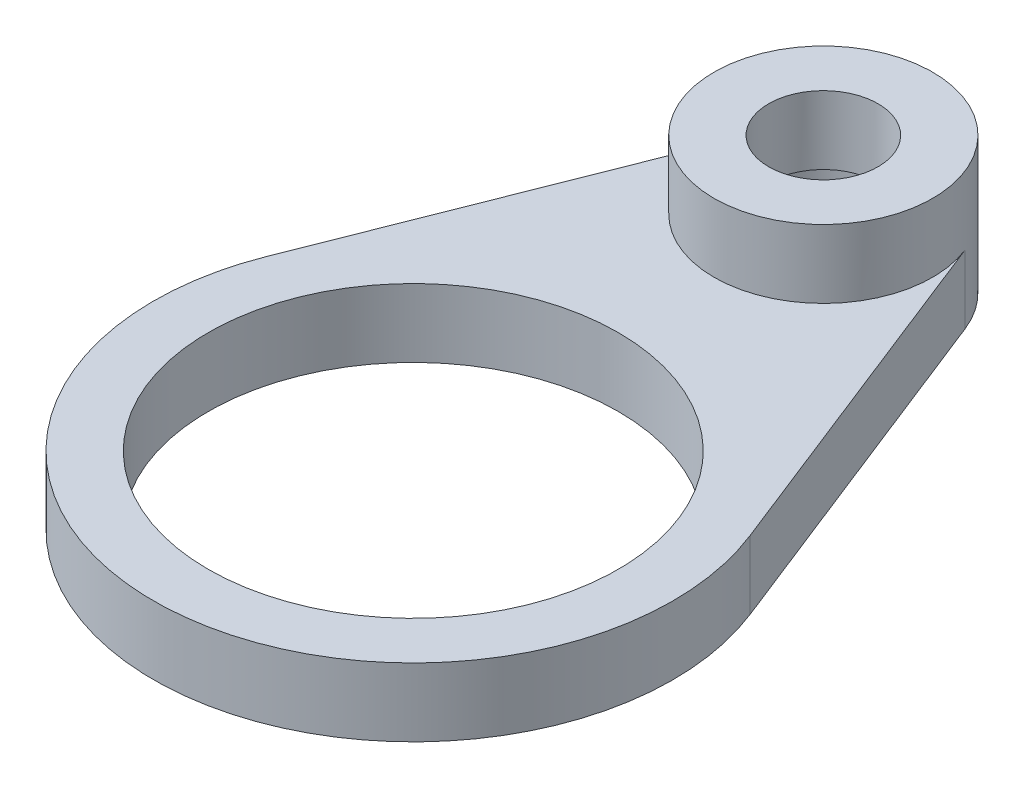
SolidWorks part; units mm, degrees
ref_plane "Front Plane" through (0, 0, 0) normal (0, 0, 1) x (1, 0, 0)
ref_plane "Top Plane" through (0, 0, 0) normal (0, 1, 0) x (1, 0, 0)
ref_plane "Right Plane" through (0, 0, 0) normal (1, 0, 0) x (0, 0, -1)
other "Configuration Table"
sketch "Sketch1" plane through (0, 0, 0) normal (0, 1, 0) x (1, 0, 0)
  line L0 (0, 0) -> (0, -30) construction
  line L1 (-7.4428, 2.9333) -> (-17.6767, -23.0333)
  line L2 (0, 25.8207) -> (0, -71.8727) construction
  line L3 (7.4428, 2.9333) -> (17.6767, -23.0333)
  arc A0 (7.4428, 2.9333) -> (-7.4428, 2.9333) centre (0, 0) ccw
  arc A1 (-17.6767, -23.0333) -> (17.6767, -23.0333) centre (0, -30) ccw
  dimension "D2" = 16
  dimension "D3" = 38
  dimension "D1" = 30
extrude "Boss-Extrude1" add sketch "Sketch1" along normal blind 5
sketch "Sketch2" plane through (0, 5, 0) normal (0, 1, 0) x (1, 0, 0)
  circle A0 centre (0, 0) radius 8
  dimension "D1" = 16
extrude "Boss-Extrude2" add sketch "Sketch2" along normal blind 5
sketch "Sketch3" plane through (0, 10, 0) normal (0, 1, 0) x (1, 0, 0)
  circle A0 centre (0, 0) radius 4
  circle A1 centre (0, -30) radius 15
  dimension "D1" = 30
  dimension "D2" = 8
extrude "Cut-Extrude1" cut sketch "Sketch3" against normal blind 39
sketch "Sketch4" plane through (0, 0, 0) normal (0, -1, 0) x (1, 0, 0)
  circle A0 centre (0, 0) radius 4.5
  dimension "D1" = 9
extrude "Cut-Extrude2" cut sketch "Sketch4" against normal blind 5
